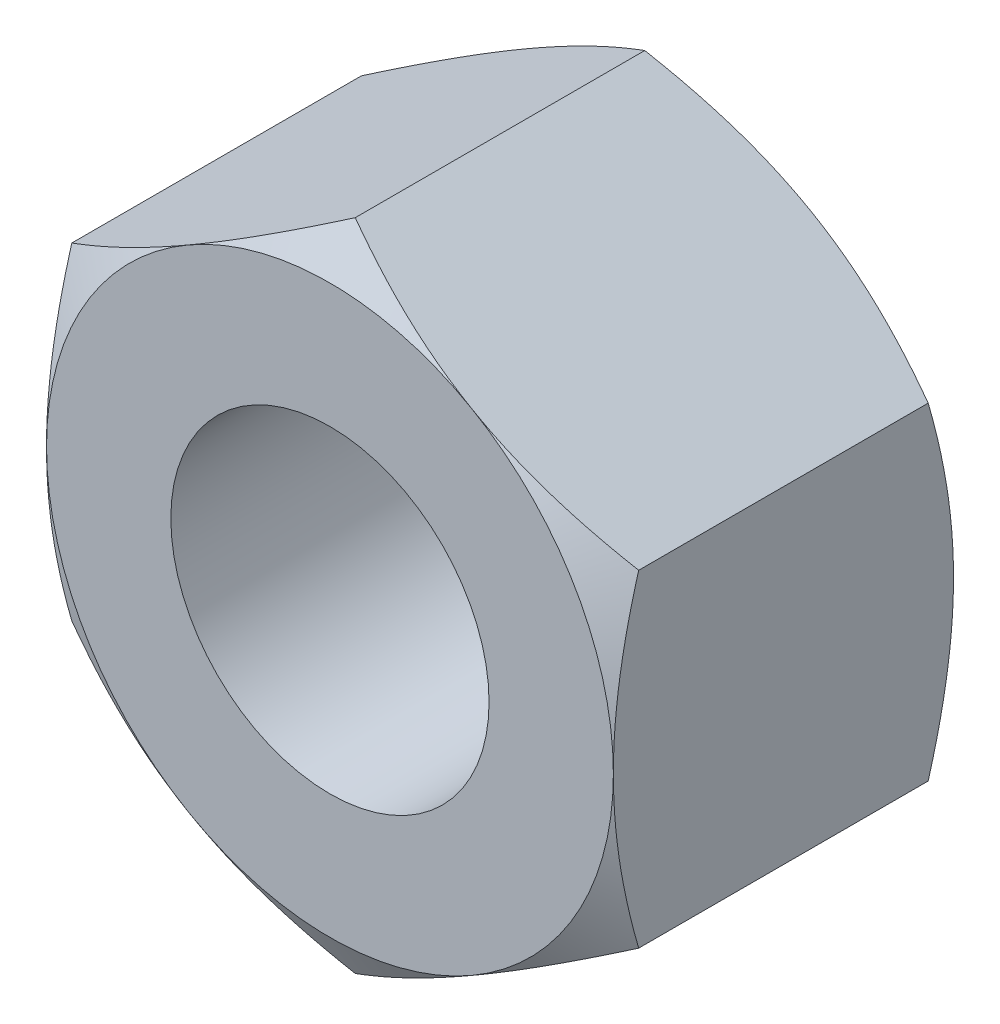
SolidWorks part; units mm, degrees
ref_plane "基准面1" through (0, 0, 0) normal (0, 0, 1) x (1, 0, 0)
ref_plane "基准面2" through (0, 0, 0) normal (0, 1, 0) x (1, 0, 0)
ref_plane "基准面3" through (0, 0, 0) normal (1, 0, 0) x (0, 0, -1)
sketch "尺寸草图" plane through (0, 0, 0) normal (0, 0, 1) x (1, 0, 0)
  line L0 (0, 0) -> (20, 0) construction
  line L1 (0, 0) -> (40, 0) construction
  line L2 (20, 0) -> (36.6, 0) construction
  line L3 (-11.4286, 0) -> (0, 0) construction
  point P3 (12, 0)
  point P4 (1.75, 0)
  point P5 (20, 0)
  point P6 (10.8, 0)
  point P8 (18, 0)
  dimension "D1" = 11.4286
  dimension "D" = 12
  dimension "P" = 1.75
  dimension "e(最小)" = 20
  dimension "m(最大)" = 10.8
  dimension "s(公称)" = 18
  dimension "dw(最小)" = 16.6
sketch "草图1" plane through (0, 0, 0) normal (0, 0, 1) x (1, 0, 0)
  line L0 (-9, 0) -> (9, 0) construction
  line L1 (0, 10.3923) -> (0, -10.3923) construction
  line L3 (0, 10.3923) -> (-9, 5.1962)
  line L4 (-9, 5.1962) -> (-9, -5.1962)
  line L5 (-9, -5.1962) -> (0, -10.3923)
  line L6 (0, -10.3923) -> (9, -5.1962)
  line L7 (9, -5.1962) -> (9, 5.1962)
  line L8 (9, 5.1962) -> (0, 10.3923)
  circle A0 centre (0, 0) radius 9 construction
  circle A1 centre (0, 0) radius 5.0528
  point P2 (0, 9.6077)
  dimension "D1" = 20
  dimension "D" = 10.1056
  dimension "D2" = 18
extrude "基体-拉伸" add sketch "草图1" along normal blind 10.8
cosmetic thread "装饰螺纹线1" parameters "D2"=12
sketch "草图2" plane through (0, 0, 0) normal (0, 0, -1) x (-1, 0, 0)
  circle A0 centre (0, 0) radius 9
  circle A1 centre (0, 0) radius 5.0528 construction
  dimension "s" = 18
extrude "切除-拉伸1" cut sketch "草图2" against normal through all draft 60 flip side to cut
sketch "草图3" plane through (0, 0, 10.8) normal (0, 0, 1) x (1, 0, 0)
  circle A0 centre (0, 0) radius 9
  dimension "D1" = 18
extrude "切除-拉伸2" cut sketch "草图3" against normal through all draft 60 flip side to cut
